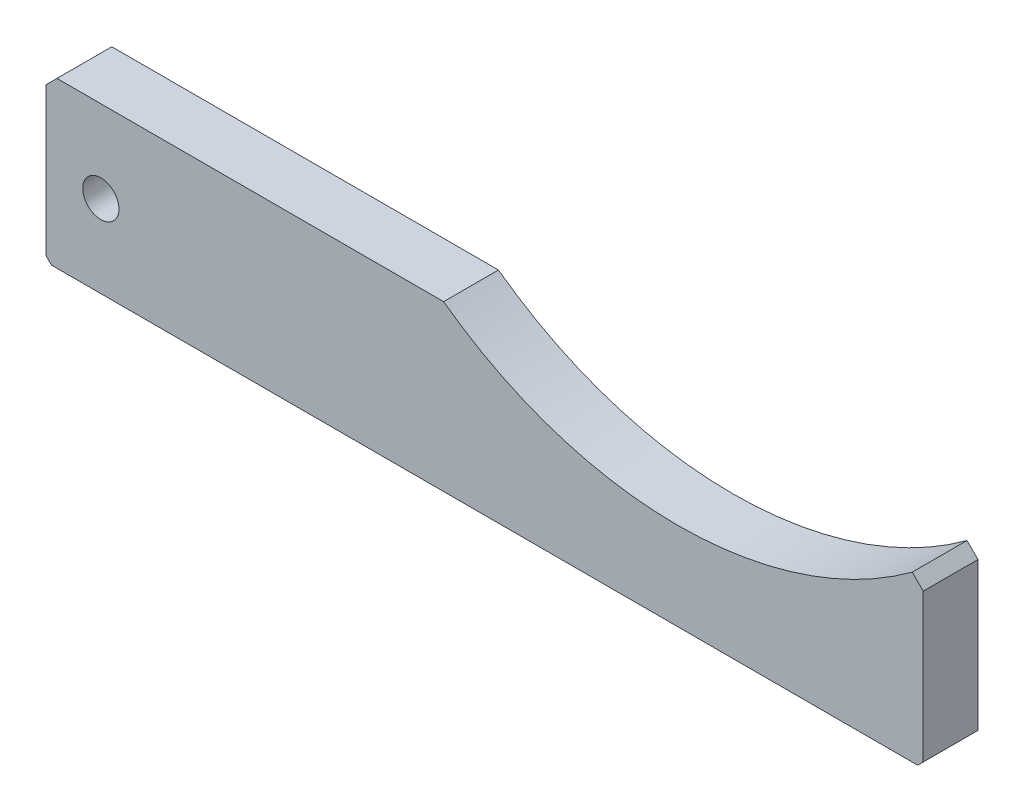
SolidWorks part; units mm, degrees
ref_plane "前视基准面" through (0, 0, 0) normal (0, 0, 1) x (1, 0, 0)
ref_plane "上视基准面" through (0, 0, 0) normal (0, 1, 0) x (1, 0, 0)
ref_plane "右视基准面" through (0, 0, 0) normal (1, 0, 0) x (0, 0, -1)
sketch "草图1" plane through (0, 0, 0) normal (0, 0, 1) x (1, 0, 0)
  line L1 (-80, -15) -> (80, -15)
  line L2 (-80, -15) -> (-80, 15)
  line L3 (-80, 15) -> (80, 15)
  line L4 (80, -15) -> (80, 15)
  line L5 (-80, -15) -> (80, 15) construction
  line L6 (-80, 15) -> (80, -15) construction
  point P0 (0, 0)
  dimension "D1" = 30
  dimension "D2" = 160
extrude "凸台-拉伸1" add sketch "草图1" along normal blind 10
chamfer "倒角1" distance 2 angle 45 2 edges at (-80, 15, 5) (80, 15, 5)
chamfer "倒角2" distance 1 angle 45 2 edges at (-80, -15, 5) (80, -15, 5)
hole_wizard "M6 间隙孔1" positions "草图2" profile "草图3" hole size "M6" standard "GB" end condition through all
sketch "草图2" plane through (0, 0, 10) normal (0, 0, 1) x (1, 0, 0)
  line L0 (-70, 0) -> (0, 0) construction
  line L2 (-80, 13) -> (-80, -14) construction
  point P0 (-70, 0)
  dimension "D1" = 10
sketch "草图3" plane through (-70, 0, 10) normal (1, 0, 0) x (0, -1, 0)
  line L0 (0, 0) -> (0, 10)
  line L1 (0, 10) -> (3.3, 10)
  line L2 (3.3, 10) -> (3.3, 0)
  line L5 (3.3, 0) -> (0, 0)
  line L11 (0, -6.35) -> (0, 107.95) construction
  dimension "通孔孔直径" = 6.6
  dimension "通孔孔深度" = 10
sketch "草图4" plane through (0, 0, 10) normal (0, 0, 1) x (1, 0, 0)
  line L0 (78, 15) -> (-78, 15) construction
  line L1 (-7.4685, 15) -> (78, 15)
  arc A0 (78, 15) -> (-7.4685, 15) centre (35.2658, 73.3102) cw
extrude "切除-拉伸1" cut sketch "草图4" against normal through all
